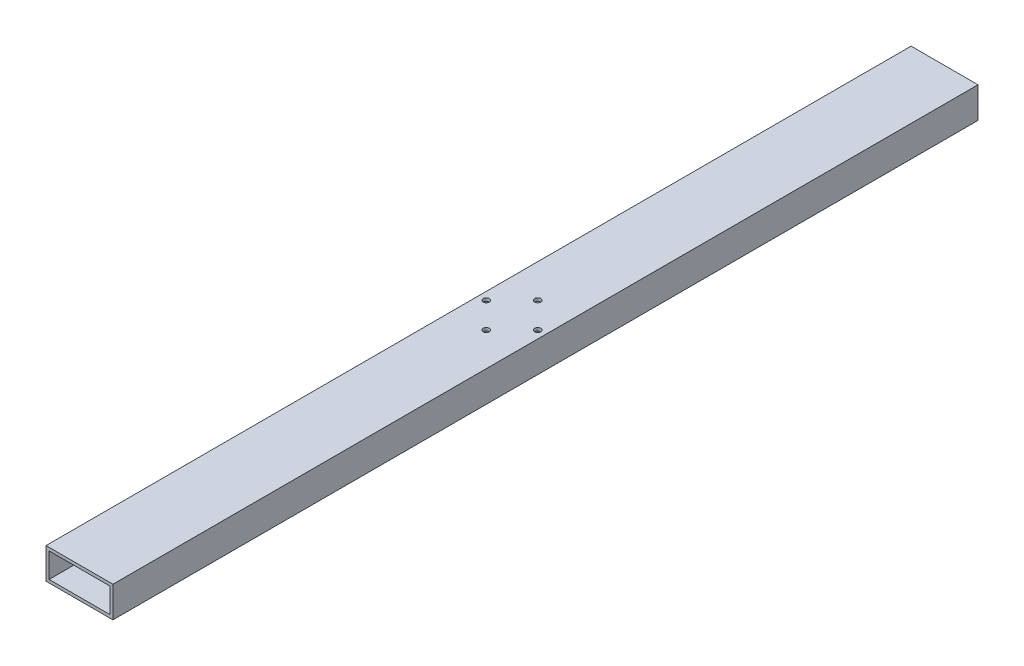
SolidWorks part; units mm, degrees
ref_plane "Front Plane" through (0, 0, 0) normal (0, 0, 1) x (1, 0, 0)
ref_plane "Top Plane" through (0, 0, 0) normal (0, 1, 0) x (1, 0, 0)
ref_plane "Right Plane" through (0, 0, 0) normal (1, 0, 0) x (0, 0, -1)
other "Configuration Table"
sketch "Sketch1" plane through (0, 0, 0) normal (0, 0, 1) x (1, 0, 0)
  line L0 (-40.5408, 39.808) -> (24.4592, 39.808)
  line L1 (24.4592, 39.808) -> (24.4592, 9.808)
  line L2 (24.4592, 9.808) -> (-40.5408, 9.808)
  line L3 (-40.5408, 9.808) -> (-40.5408, 39.808)
extrude "Boss-Extrude1" add sketch "Sketch1" along normal blind 840
sketch "Sketch2" plane through (0, 0, 840) normal (0, 0, 1) x (1, 0, 0)
  line L0 (-37.5408, 36.808) -> (21.4592, 36.808)
  line L1 (21.4592, 36.808) -> (21.4592, 12.808)
  line L2 (21.4592, 12.808) -> (-37.5408, 12.808)
  line L3 (-37.5408, 12.808) -> (-37.5408, 36.808)
  line L4 (24.4592, 39.808) -> (-40.5408, 39.808) construction
  line L5 (24.4592, 9.808) -> (24.4592, 39.808) construction
  line L6 (-40.5408, 9.808) -> (24.4592, 9.808) construction
  line L7 (-40.5408, 39.808) -> (-40.5408, 9.808) construction
  dimension "D1" = 3
  dimension "D2" = 3
  dimension "D3" = 3
  dimension "D4" = 3
extrude "Cut-Extrude1" cut sketch "Sketch2" against normal blind 950
sketch "Sketch3" plane through (0, 39.808, 0) normal (0, 1, 0) x (1, 0, 0)
  line L0 (-8.0408, 0) -> (-8.0408, -39.0581) construction
  line L1 (24.4592, 0) -> (-40.5408, 0) construction
  circle A0 centre (-8.0408, -39.0581) radius 9.584
sketch "Sketch5" plane through (0, 9.808, 0) normal (0, -1, 0) x (-1, 0, 0)
  line L0 (33.0408, -420) -> (30.0408, -420) construction
  line L1 (-13.9592, -420) -> (-16.9592, -420) construction
  circle A1 centre (8.0408, -395) radius 3
  circle A2 centre (33.0408, -420) radius 3
  circle A3 centre (8.0408, -445) radius 3
  circle A4 centre (-16.9592, -420) radius 3
  dimension "D2" = 6
  dimension "D3" = 6
  dimension "D4" = 6
  dimension "D5" = 6
extrude "Cut-Extrude3" cut sketch "Sketch5" against normal through all
